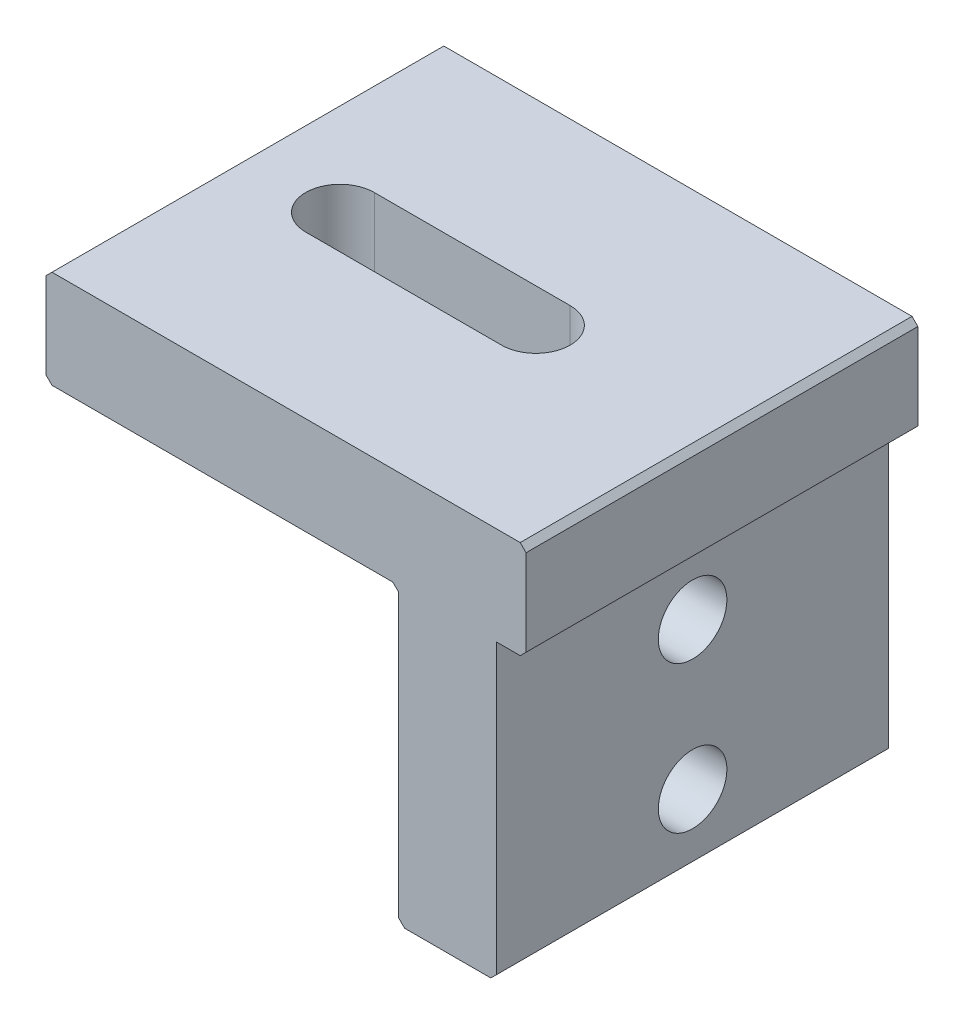
from build123d import *

# Parameters (mm, degrees)
BOSS_EXTRUDE1_DEPTH = 20
CUT_EXTRUDE2_REACH  = 35.971
SKETCH2_R           = 1.75
CUT_EXTRUDE3_REACH  = 37.004


with BuildPart() as part:
    # Sketch1 → Boss-Extrude1 (new body)
    with BuildSketch(Plane.XY):
        Polygon((-6.8, 0), (-24.2, 0), (-24.5, 0.3), (-24.5, 4.7), (-24.2, 5), (-0.3, 5), (0, 4.7), (0, 0.3), (-0.3, 0), (-1.5, 0), (-1.5, -14.7), (-1.8, -15), (-6.2, -15), (-6.5, -14.7), (-6.5, -0.3), align=None)
    extrude(amount=BOSS_EXTRUDE1_DEPTH)

    # Sketch2 → Cut-Extrude2 (cut, up to next)
    with BuildSketch(Plane(origin=(-1.5, 0, 0), x_dir=(0, 0, -1), z_dir=(1, 0, 0)), mode=Mode.PRIVATE) as cut_extrude2_sk1:
        with Locations(Location((-10, -11.5, 0), (0, 0, 90))):
            Circle(SKETCH2_R)
    cut_extrude2_tool1 = extrude(cut_extrude2_sk1.sketch, amount=-CUT_EXTRUDE2_REACH, mode=Mode.PRIVATE) & part.part
    # Sketch2 → Cut-Extrude2 (cut, up to next)
    with BuildSketch(Plane(origin=(-1.5, 0, 0), x_dir=(0, 0, -1), z_dir=(1, 0, 0)), mode=Mode.PRIVATE) as cut_extrude2_sk2:
        with Locations(Location((-10, -4, 0), (0, 0, 90))):
            Circle(SKETCH2_R)
    cut_extrude2_tool2 = extrude(cut_extrude2_sk2.sketch, amount=-CUT_EXTRUDE2_REACH, mode=Mode.PRIVATE) & part.part
    add(cut_extrude2_tool1.solids().sort_by_distance((-1.5, -11.5, 10))[0], mode=Mode.SUBTRACT)
    add(cut_extrude2_tool2.solids().sort_by_distance((-1.5, -4, 10))[0], mode=Mode.SUBTRACT)

    # Sketch5 → Cut-Extrude3 (cut, up to next)
    with BuildSketch(Plane.XZ, mode=Mode.PRIVATE) as cut_extrude3_sk1:
        with BuildLine():
            Line((-19.5, 11.75), (-9.5, 11.75))
            ThreePointArc((-9.5, 11.75), (-7.75, 10), (-9.5, 8.25))
            Line((-9.5, 8.25), (-19.5, 8.25))
            ThreePointArc((-19.5, 8.25), (-21.25, 10), (-19.5, 11.75))
        make_face()
    cut_extrude3_tool1 = extrude(cut_extrude3_sk1.sketch, amount=-CUT_EXTRUDE3_REACH, mode=Mode.PRIVATE) & part.part
    add(cut_extrude3_tool1.solids().sort_by_distance((-14.5, 0, 10))[0], mode=Mode.SUBTRACT)


solid = part.part
